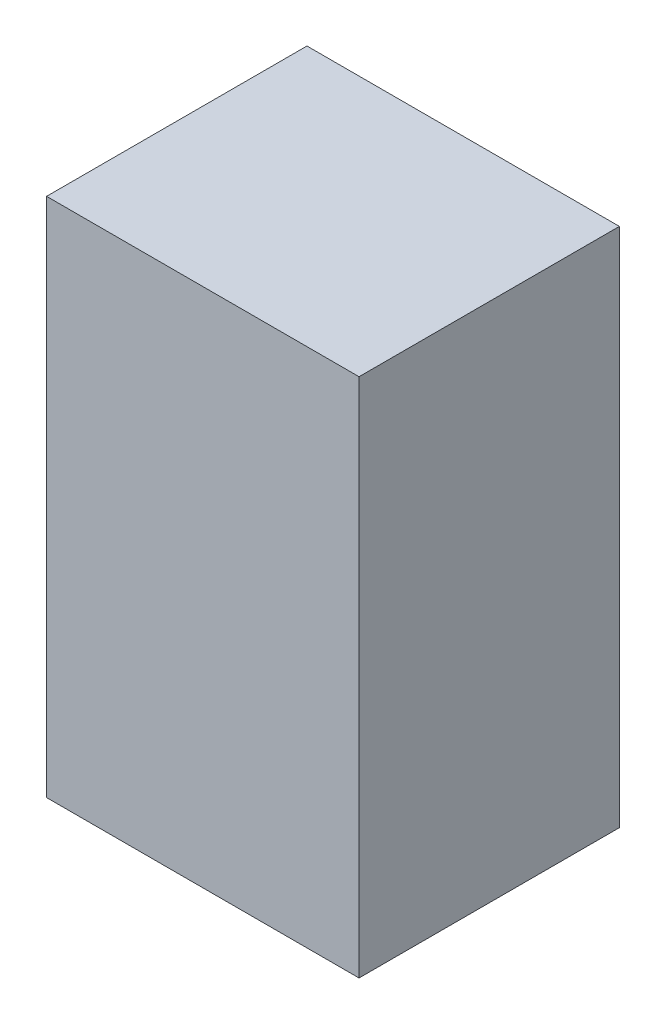
SolidWorks part; units mm, degrees
ref_plane "Front Plane" through (0, 0, 0) normal (0, 0, 1) x (1, 0, 0)
ref_plane "Top Plane" through (0, 0, 0) normal (0, 1, 0) x (1, 0, 0)
ref_plane "Right Plane" through (0, 0, 0) normal (1, 0, 0) x (0, 0, -1)
other "Configuration Table"
sketch "Sketch1" plane through (0, 0, 0) normal (0, 0, 1) x (1, 0, 0)
  line L13 (0, 0) -> (30, 0)
  line L14 (0, 0) -> (0, 50)
  line L15 (0, 50) -> (30, 50)
  line L16 (30, 0) -> (30, 50)
  dimension "D1" = 30
  dimension "D2" = 50
extrude "Boss-Extrude1" add sketch "Sketch1" along normal blind 25
